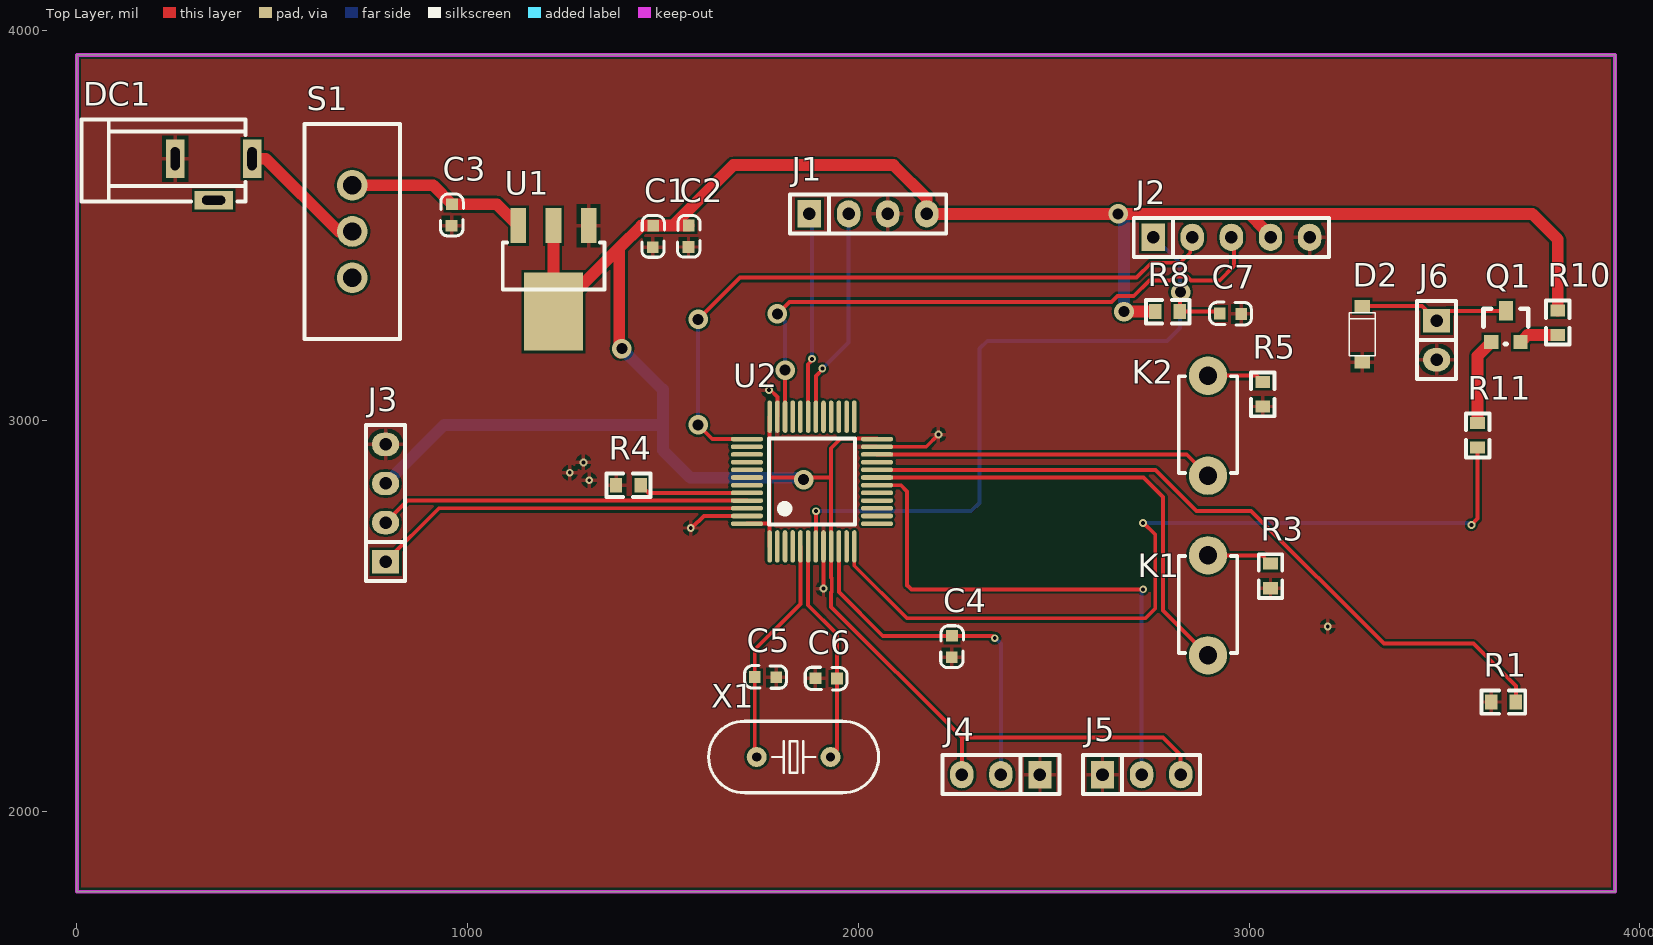
[diagram p0: Top Layer view]
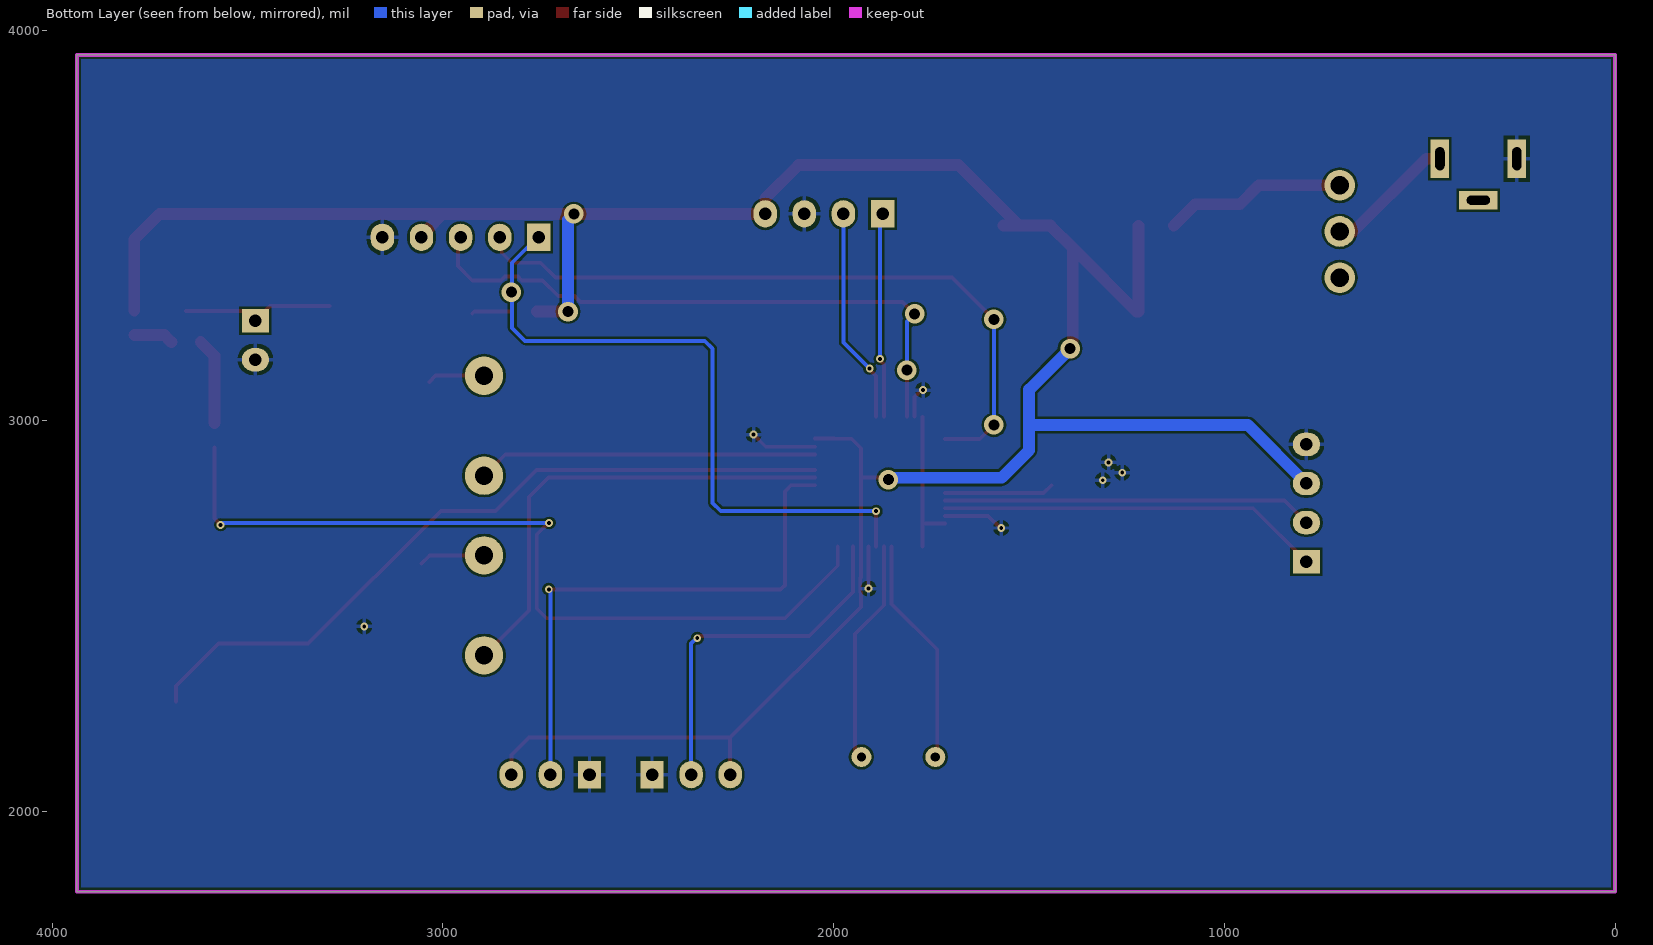
[diagram p1: Bottom Layer view, seen from below]
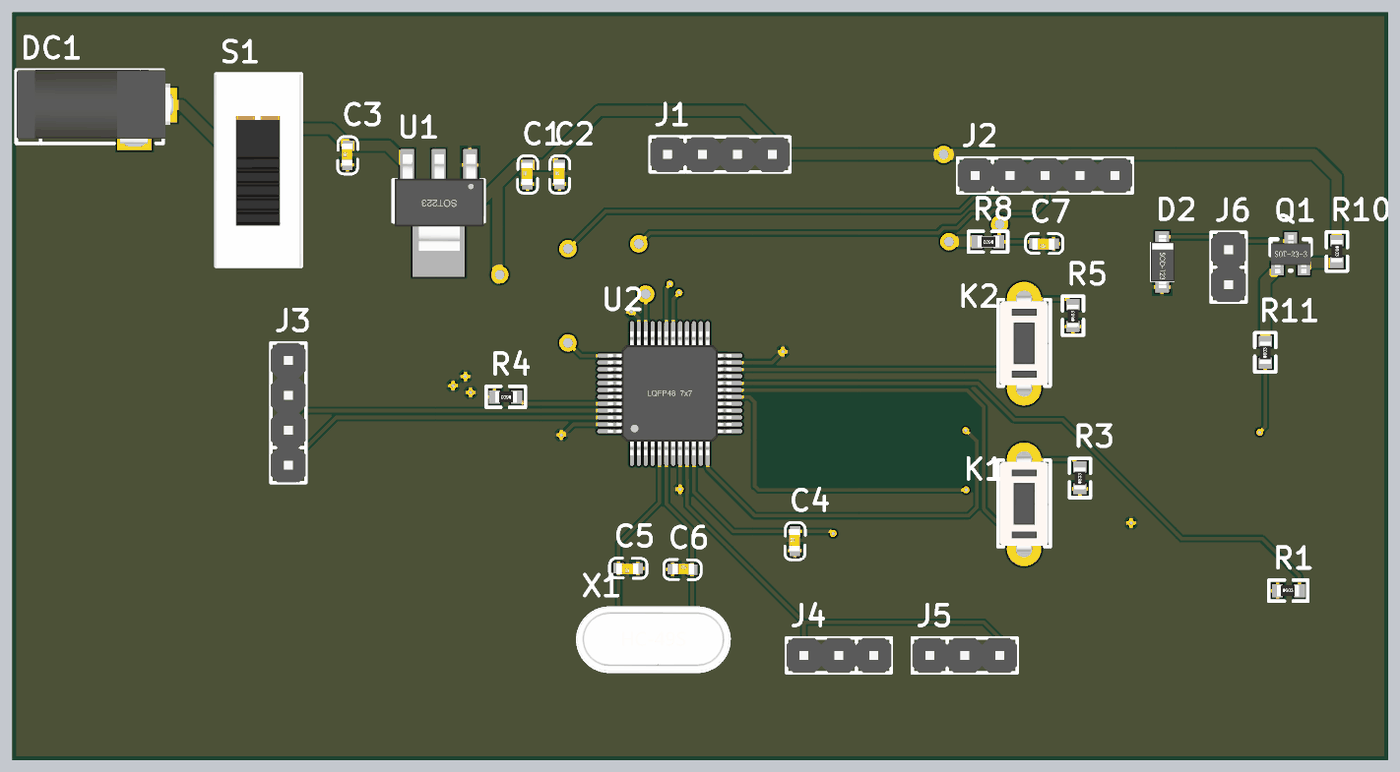
[diagram p2: 3D render of the assembled board from above, using the file's embedded part models]
# Altium PCB MISC82702.PcbDoc
Units mil, origin at the board's own origin, x right, y up, seen from the top; angles counter-clockwise.
Board outline 3937.01 x 2142.01 mil, 2 copper layers (Top Layer, Bottom Layer); 29 components, 25 nets, 118 pads, 24 vias.

## Layer stack, top to bottom (the 12.6 mil dielectric is the usual default, probably not edited)
Top Solder: solder mask 0.4, Solder Resist, Dk 3.5
Top Layer: signal copper 1.4
Dielectric 1: dielectric 12.6, FR-4, Dk 4.8
Bottom Layer: signal copper 1.4
Bottom Solder: solder mask 0.4, Solder Resist, Dk 3.5

## Board outline
0,1795 3937.01,1795 3937.01,3937.01 0,3937.01

## Design rules (kind name [scope] priority, off if disabled: settings)
Clearance [All] p1: gap=6 except(0: Arc-Text Track-Text SMDPad-Text THPad-Text Via-Text Fill-Text Poly-Text Region-Text Text-Text)
MinimumSolderMaskSliver [All] p1: minsoldermaskwidth=0
PolygonConnect [All] p1: connectstyle=Relief reliefconductorwidth=10 reliefentries=4 polygonreliefangle="90 Angle" airgapwidth=10
RoutingVias [All] p1: holewidth=10 width=20 viastyle="Through Hole" minholewidth=10 minwidth=20 maxholewidth=10 maxwidth=50
SilkToSilkClearance [All] p1: silktosilkclearance=0
SilkToSolderMaskClearance [IsPad] p1: minsilkscreentomaskgap=0 clearancetoexposedcopper=TRUE
SolderMaskExpansion [All] p1: expansion=4
Width [All] p1: maxlimit=50 minlimit=10 preferedwidth=10
27 further rules are at their usual default settings.

## Components (designator, comment, footprint, x,y, rotation, side; value= is the part's Value field where it differs from the comment)
C1 "10uF" 0603C 1473.65,3444.79 r90 top
C2 "0.1uF" 0603C 1565,3445 r90 top
C3 "10uF" 0603C 958.65,3499.79 r90 top
C4 "0.1uF" 0603C 2238.65,2394.79 r90 top
C5 "20pF" 0603C 1790.21,2343.65 r180 top
C6 "20pF" 0603C 1890,2342.01 r0 top
C7 "0.1uF" 0603C 2980.21,3273.65 r180 top
D2 "DIODE" SOD-123 3290,3152.01 r90 top
DC1 "DC_Socket" DC-002 448.43,3671.3 r180 top
J1 "Pin HDR1X4" "Pin HDR1X4/2.54mm-S" 1875,3530 r90 top
J2 "Pin HDR1X5" "Pin HDR1X5/2.54mm-S" 2755,3470 r90 top
J3 "Pin HDR1X4" "Pin HDR1X4/2.54mm-S" 790,2640 r180 top
J4 "Pin HDR1X3" "Pin HDR1X3/2.54mm-S" 2465,2095 r270 top
J5 "Pin HDR1X3" "Pin HDR1X3/2.54mm-S" 2625,2095 r90 top
J6 "Pin HDR1X2" "Pin HDR1X2/2.54mm-S" 3480,3257.01 r0 top
K1 "KEY" DIP-3X6X4.3 2895,2400 r90 top
K2 "KEY" DIP-3X6X4.3 2895,2860 r90 top
Q1 "PNP" SOT-23 3655,3237.01 r0 top
R1 "10K" 0603R 3620,2280.65 r0 top
R3 "10K" 0603R 3055,2572.01 r90 top
R4 "10K" 0603R 1442.99,2835.63 r180 top
R5 "10K" 0603R 3035,3037.01 r90 top
R8 "10K" 0603R 2822.99,3280 r180 top
R10 "470" 0603R 3790,3282.99 r270 top
R11 "470" 0603R 3585,2932.01 r90 top
S1 "SS-12D10" SS-12D10 705,3603.11 r270 top
U1 "AMS1117" SOT223 1220,3500 r180 top
U2 "STM32F103C8T6" "LQFP48 7X7" 1881.42,2845.47 r0 top
X1 "XTAL-2P" "OSC HC-49S" 1834.49,2140 r0 top

## Footprints (in the part's own frame and the unit in brackets; to place one, negate y for a bottom-side part, rotate by r counter-clockwise, add the part's x,y. Pads: shape width x height; smd on the part's side, far side on the other; paste and mask are expansions set on the pad)
0603C [mil]
  rect 30x30 smd: 1(0.21,-0.35) 2(55.21,-1.35)
  silkscreen extent -26,-30 81,28, body extent -1,-15 62,17, height 12
0603R [mm]
  rect 0.8x0.965 smd: 1(0,0) 2(1.6,0)
  silkscreen extent -0.64,-0.76 2.21,0.76, body extent -0.04,-0.41 1.56,0.41, height 0.45
DC-002 [mm] "3.5X1.1mm"
  rect 1.2x2.5 hole 0.6 slot 1.5 at 90 deg: 1(0,0) 2(5,0)
  rect 2.5x1.2 hole 0.6 slot 1.5 at 0 deg: 3(2.5,2.7)
  silkscreen extent 0.43,-2.54 11.1,2.79, body extent -0.25,-2.55 11.05,2.8, height 7.3
DIP-3X6X4.3 [mm]
  round 2.5 hole 1.2: 1(0,0) 3(6.5,0)
  silkscreen extent 0.16,-1.9 6.46,1.9, body extent -0.64,-1.75 7.19,1.75, height 4.31
"LQFP48 7X7" [mm]
  oval 0.3x2.1 smd: 1(-2.75,-4.227) 2(-2.25,-4.227) 3(-1.75,-4.227) 4(-1.25,-4.227) 5(-0.75,-4.227) 6(-0.25,-4.227) 7(0.25,-4.227) 8(0.75,-4.227) 9(1.25,-4.227) 10(1.75,-4.227) 11(2.25,-4.227) 12(2.75,-4.227) 25(2.75,4.202) 26(2.25,4.202) 27(1.75,4.202) 28(1.25,4.202) 29(0.75,4.202) 30(0.25,4.202) 31(-0.25,4.202) 32(-0.75,4.202) 33(-1.25,4.202) 34(-1.75,4.202) 35(-2.25,4.202) 36(-2.75,4.202)
  oval 2.1x0.3 smd: 13(4.227,-2.75) 14(4.227,-2.25) 15(4.227,-1.75) 16(4.227,-1.25) 17(4.227,-0.75) 18(4.227,-0.25) 19(4.227,0.25) 20(4.227,0.75) 21(4.227,1.25) 22(4.227,1.75) 23(4.227,2.25) 24(4.227,2.75) 37(-4.227,2.75) 38(-4.227,2.25) 39(-4.227,1.75) 40(-4.227,1.25) 41(-4.227,0.75) 42(-4.227,0.25) 43(-4.227,-0.25) 44(-4.227,-0.75) 45(-4.227,-1.25) 46(-4.227,-1.75) 47(-4.227,-2.25) 48(-4.227,-2.75)
  silkscreen extent -2.79,-2.79 2.79,2.79, body extent -4.51,-4.5 4.5,4.5, height 1.45
"OSC HC-49S" [mm]
  round 1.3 hole 0.6: 1(-2.4,0) 2(2.4,0)
  silkscreen extent -5.52,-2.32 5.52,2.33, body extent -5.53,-2.29 5.53,2.36, height 4.13
"Pin HDR1X2/2.54mm-S" [mil]
  rect 70x60 hole 32: 1(0,0)
  oval 70x60 hole 32: 2(0,-100)
  silkscreen extent -50,-150 50,50, body extent -50,-150 50,50, height 336
"Pin HDR1X3/2.54mm-S" [mil]
  rect 70x60 hole 32: 1(0,0)
  oval 70x60 hole 32: 2(0,-100) 3(0,-200)
  silkscreen extent -50,-250 50,50, body extent -50,-250 50,50, height 336
"Pin HDR1X4/2.54mm-S" [mil]
  rect 70x60 hole 32: 1(0,0)
  oval 70x60 hole 32: 2(0,-100) 3(0,-200) 4(0,-300)
  silkscreen extent -50,-350 50,50, body extent -50,-350 50,50, height 336
"Pin HDR1X5/2.54mm-S" [mil]
  rect 70x60 hole 32: 1(0,0)
  oval 70x60 hole 32: 2(0,-100) 3(0,-200) 4(0,-300) 5(0,-400)
  silkscreen extent -50,-450 50,50, body extent -50,-450 50,50, height 336
SOD-123 [mm] "塑封二极管"
  rect 0.8x1 smd: A(-0.051,0) K(3.607,0)
  silkscreen extent 0.38,-0.85 3.18,0.85, body extent -0.12,-0.89 3.73,0.81, height 1.43
SOT223 [mil]
  rect 40x90 smd: 1(-90,0) 2(0,0) 3(90,0)
  rect 150x200 smd: 2(0,220)
  silkscreen extent -130,43 130,163, body extent -130,-30 126,246, height 65
SOT-23 [mil]
  rect 36x36 smd: B(-35,-35) E(40,-35)
  rect 36x50 smd: C(3,45)
  silkscreen extent -55,-40 60,50, body extent -54,-48 60,62, height 47
SS-12D10 [mm]
  round 2 hole 1.2: 1(0,0) 2(3,0) 3(6,0)
  silkscreen extent -4,-3.1 10,3.1, body extent -3.95,-3.15 10.05,3.05, height 9.65

## Part data
C1 C2 C3 C4 C5 C6 C7: library part CAP, "Non-polar capacitor"
D2: "General-purpose diode"
Q1: "PNP transistor"
R1 R3 R4 R5 R8 R10 R11: library part RES
U1: "Three-terminal voltage regulator"
X1: "2-pin passive crystal oscillator"

## Via types
v1: diameter 20, hole 10, Top Layer to Bottom Layer, 15 vias
v2: diameter 50, hole 28, Top Layer to Bottom Layer, 9 vias

## Nets (pads, with @x,y where several pads share a name; then routed paths per layer and width w, separated by ;. In a path a pad name is that pad's centre, name@x,y a point inside that pad or via, vN(x,y) a via of type N, cw(c..) or ccw(c..) an arc to the next point about the centre after c; other vN are vias at no path point)
+5: C3.2 S1.1 U1.3 | length 467.7
  Top Layer w30: S1.1 911.89,3603.11 C3.2 1075,3555 U1.3
adc1: C4.2 J4.2 U2.10 | length 920.8
  Top Layer w10: U2.10 1950.32,2562.23 2062.54,2450 C4.2 2343.27,2450 v1(2349.14,2444.14)
  Bottom Layer w10: v1@2350,2445 2365,2430 J4.2
boot: R4.1 U2.44 | length 280.2
  Top Layer w10: R4.1 1462.68,2815.95 U2.44
GND: C1.1 C2.1 C3.1 C4.1 C5.1 C6.1 C7.1 D2.A DC1.2 J1.3 J2.5 J3.4 J4.1 J5.1 J6.2 R1.1 R3.1 R4.2 R5.1 U1.1 U2.8 U2.23 U2.35 U2.47 | length 507.4
  Top Layer w10: v1@1574.76,2727.04 1604.6,2756.89 U2.47 ; v1@1774.67,3080 1792.83,3061.84 U2.35 ; v1(1910.94,2570.93) U2.8 ; U2.23 2173.85,2934.06 v1(2205,2965.21)
  other v1: 3201.42,2474.14 1571.17,2726.18 1311.42,2848.25 1261.42,2867.67 1296.42,2894.14 1771.09,3079.14
ir_ext: J5.2 U2.18 | length 1410.6
  Top Layer w10: U2.18 2109.37,2835.63 2125,2820 2124.14,2819.14 2124.14,2579.14 ; 2125,2580 2135.86,2569.14 v1(2729.14,2569.14)
  Bottom Layer w10: J5.2 2725,2565 v1(2729.14,2569.14) v1@2730,2570
mcu_key1: K1.1 U2.19 | length 1206
  Top Layer w10: U2.19 2730.31,2855.32 2780.16,2805.47 2780.16,2514.84 K1.1
mcu_key2: K2.1 U2.22 | length 869.7
  Top Layer w10: U2.22 2840.63,2914.37 K2.1
NetD2_K: D2.K J6.1 Q1.C | length 393.7
  Top Layer w10: D2.K 3443,3294.01 J6.1 3505,3282.01 Q1.C
NetDC1_1: DC1.1 S1.2 | length 333.7
  Top Layer w30: DC1.1 483.7,3671.3 670,3485 S1.2
NetK1_3: K1.3 R3.2 | length 169.2
  Top Layer w10: K1.3 3035,2655.91 3035,2655 R3.2
NetK2_3: K2.3 R5.2 | length 146.6
  Top Layer w10: K2.3 3019.09,3115.91 R5.2
NetQ1_B: Q1.B R11.2 | length 221.5
  Top Layer w30: R11.2 3585,3167.01 Q1.B
NetQ1_E: Q1.E R10.2 | length 102.5
  Top Layer w30: Q1.E 3712.99,3220 R10.2
NetR1_2: R1.2 U2.20 | length 1904.2
  Top Layer w10: U2.20 2760.95,2875 2865.95,2770 3005,2770 3345,2430 3575,2430 3682.99,2322.01 R1.2@3682.99,2282.01
nrst: C7.2 J2.1 R8.1 U2.7 | length 1866.5
  Top Layer w10: U2.7 1891.26,2766.26 v1@1895,2770 ; v2(2825,3330) 2822.99,3327.99 R8.1 2920,3280 C7.2
  Bottom Layer w10: v1(1891.42,2769.14) 2289.14,2769.14 2310,2790 2310,3185 2330,3205 2790,3205 2822.99,3237.99 2822.99,3405 2757.99,3470 J2.1
oled_scl: J3.2 U2.45 | length 948.3
  Top Layer w10: J3.2 846.26,2796.26 U2.45
oled_sda: J3.1 U2.46 | length 981.6
  Top Layer w10: J3.1 926.57,2776.57 U2.46
osc_in: C5.2 U2.5 X1.1 | length 589.5
  Top Layer w10: X1.1 1735,2145 C5.2 1735,2415 1851.89,2531.89 U2.5
osc_out: C6.2 U2.6 X1.2 | length 576.3
  Top Layer w10: U2.6 1871.57,2528.43 1945.21,2454.79 C6.2 1945.21,2156.24 X1.2
pwm: R11.1 U2.12 | length 2166.6
  Top Layer w10: U2.12 1989.69,2629.45 2124.14,2495 2735,2495 2760,2520 2760,2709.14 v1@2729.14,2740 ; v1(3569.14,2734.14) 3585,2750 R11.1
  Bottom Layer w10: v1(2728.27,2739.14) 3565.86,2739.14 v1@3570,2735
swclk: J2.2 U2.37 | length 1781.9
  Top Layer w10: v2(1590,2990) 1626.26,2953.74 U2.37 ; v2(1590,3260) 1696.89,3366.89 2711.89,3366.89 2750,3405 2824.05,3405 2849.52,3430.48 2849.52,3464.52 J2.2
  Bottom Layer w10: v2(1590,2990) v2(1590,3260)
swdio: J2.3 U2.34 | length 1567.4
  Top Layer w10: v2(1792.83,3274) 1823.83,3305 2648.43,3305 2663.43,3320 2705,3320 2745,3360 2798.43,3360 2808.43,3370 2841.57,3370 2851.57,3360 2925,3360 2961.26,3396.26 J2.3@2961.26,3465 ; U2.34 v2(1812.52,3130)
  Bottom Layer w10: v2(1792.83,3274) 1812.52,3254.31 v2(1812.52,3130)
uart_spk_rx: J1.1 U2.31 | length 521.7
  Top Layer w10: U2.31 1871.57,3145.16 v1@1881.42,3155
  Bottom Layer w10: J1.1 1881.42,3523.58 v1(1881.42,3159.14)
uart_spk_tx: J1.2 U2.30 | length 556.1
  Top Layer w10: U2.30 1891.26,3114.79 v1@1911.47,3135
  Bottom Layer w10: v1(1907.89,3134.14) 1975,3201.25 J1.2
VCC: C1.2 C2.2 J1.4 J2.4 J3.3 J4.3 J5.3 R8.2 R10.1 U1.2 U2.1 U2.9 U2.24 U2.36 U2.48 | length 7690
  Top Layer w10: U2.48 1770.35,2737.2 1773.15,2740 ; U2.1 1773.15,2740 ; U2.36 1773.15,2855 ; U2.24@2047.83,2954.96 1998.76,2954.96 1998.35,2954.55 1954.87,2954.55 1930.63,2930.31 1930.63,2855 ; J4.3 2265,2190 ; J5.3 2825,2145 2780,2190 2265,2190 ; 1773.15,2740 1773.15,2855 ; 1773.15,2855 1930.63,2855 ; 1930.63,2855 U2.9 1930.63,2599.37 1931.94,2598.06 1931.94,2562.23 1930.63,2560.91 1930.63,2524.37 2265,2190
  Top Layer w30: U1.2@1220,3500 1220,3280 1225,3280 1388.44,3443.44 ; v2@1390,3174.96 1388.44,3176.52 1388.44,3443.44 ; C2.2 1525,3500.21 ; v2(2680,3280) R8.2 ; J2.4@3040,3465 3040,3490 3000,3530 ; R10.1 3790,3465 3725,3530 3000,3530 ; 1388.44,3443.44 1445.21,3500.21 1525,3500.21 ; 1525,3500.21 1679.79,3655 2090,3655 2175,3570 J1.4 v2(2665,3530) 3000,3530
  Bottom Layer w30: J3.3 940,2990 1500,2990 ; v2(1395,3185.3) 1500,3080.3 1500,2990 ; v2@1847.82,2855 1570,2855 1500,2925 1500,2990 ; v2(2665,3530) 2680,3515 v2(2680,3280)
  other v2: 1860,2850
pads on no net: DC1.3 S1.3 U2.2 U2.3 U2.4 U2.11 U2.13 U2.14 U2.15 U2.16 U2.17 U2.21 U2.25 U2.26 U2.27 U2.28 U2.29 U2.32 U2.33 U2.38 U2.39 U2.40 U2.41 U2.42 U2.43

## Polygon pours and split planes (outlines as drawn)
GND on Top Layer "G" (solid, remove dead copper, pour order 10): -285,4155 -265,4175 4395,4175 4395,1780 3905,1290 3550,1645 -705,1645
GND on Bottom Layer "G" (solid, remove dead copper, pour order 12): -595,4205 4555,4205 4675,4085 4225,3635 4225,825 -495,825 -1115,1445

## Keep-outs
Keep-Out Layer:
  the board outline again, w10